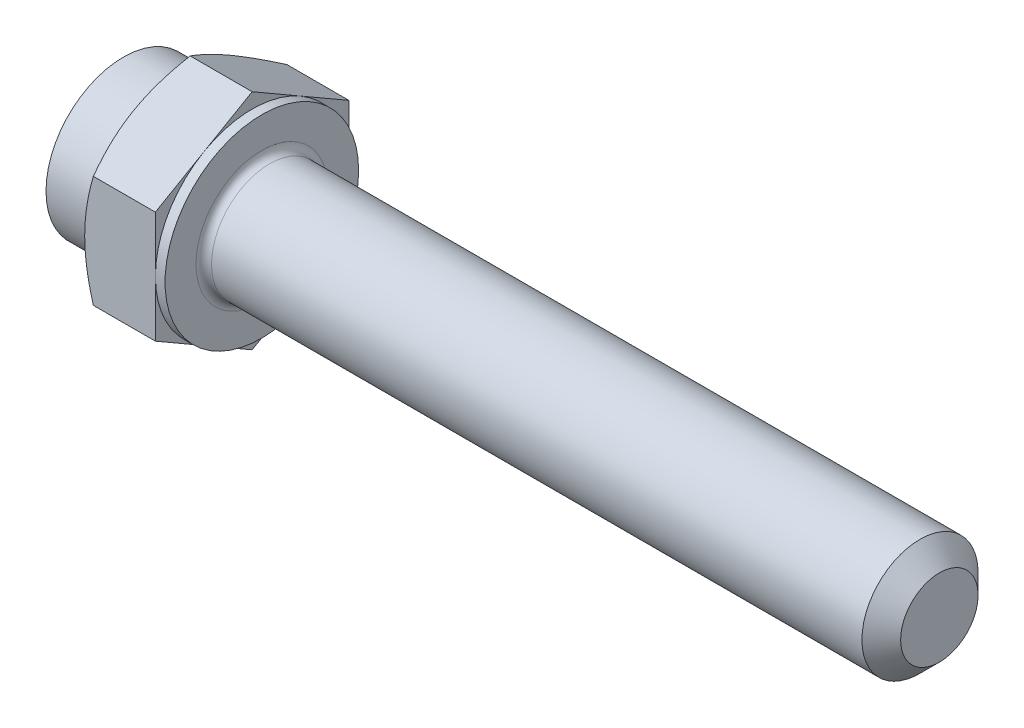
from build123d import *

# Parameters (mm, degrees)
EXTRUDE_371_DEPTH   = 4.15
SKETCH_4_W          = 0.5
SKETCH_4_H          = 10.773502692
CHAMFER_1937_SIZE   = 1
FILLET_1988_R       = 0.4
SKETCH_7_R          = 4
CUT_EXTRUDE_1_DEPTH = 3
SKETCH_8_R          = 4
EXTRUDE_1_DEPTH     = 6


with BuildPart() as part:
    # 草图1 → Extrude 371 (new body)
    with BuildSketch(Plane(origin=(0, 0, 0), x_dir=(0, 0, -1), z_dir=(1, 0, 0))):
        Polygon((5, 2.886751346), (5, -2.886751346), (0, -5.773502692), (-5, -2.886751346), (-5, 2.886751346), (0, 5.773502692), align=None)
    extrude(amount=EXTRUDE_371_DEPTH)

    # 草图2 → 凸台-旋转1 (revolve)
    with BuildSketch(Plane.XY, mode=Mode.PRIVATE) as revolve_1_sk:
        Polygon((0, 0), (39.15, 0), (39.15, 1.9175), (39.15, 3), (0, 3), align=None)
    revolve(revolve_1_sk.sketch.rotate(Axis((0, 0, 0), (1, 0, 0)), 90), axis=Axis((0, 0, 0), (1, 0, 0)))

    # 草图3 → 切除-旋转1 (revolve, cut)
    with BuildSketch(Plane.XY):
        Polygon((0, 5), (3.333333333, 10.773502692), (3.333333333, 15.773502692), (-10, 15.773502692), (-10, 5), align=None)
    revolve(axis=Axis((0, 0, 0), (1, 0, 0)), mode=Mode.SUBTRACT)

    # 草图5 → 切除-旋转2 (revolve, cut)
    with BuildSketch(Plane.XY):
        Polygon((4.15, 5), (0.816666667, 10.773502692), (0.816666667, 15.773502692), (10.816666667, 15.773502692), (10.816666667, 5), align=None)
    revolve(axis=Axis((0, 0, 0), (1, 0, 0)), mode=Mode.SUBTRACT)

    # 草图4 → 切除-旋转3 (revolve, cut)
    with BuildSketch(Plane.XY, mode=Mode.PRIVATE) as cut_revolve_3_sk:
        with Locations((3.9, 10.386751346)):
            Rectangle(SKETCH_4_W, SKETCH_4_H)
    revolve(cut_revolve_3_sk.sketch.rotate(Axis((0, 0, 0), (1, 0, 0)), 270), axis=Axis((0, 0, 0), (1, 0, 0)), mode=Mode.SUBTRACT)

    # Chamfer 1937
    chamfer_1937_edges = [part.edges().sort_by_distance(p)[0] for p in [
        (39.15, 0, -3),
    ]]
    chamfer(chamfer_1937_edges, length=CHAMFER_1937_SIZE)

    # Fillet 1988
    fillet_1988_edges = [part.edges().sort_by_distance(p)[0] for p in [
        (4.15, 0, -3),
    ]]
    fillet(fillet_1988_edges, radius=FILLET_1988_R)

    # 草图7 → 切除-拉伸1 (cut)
    with BuildSketch(Plane.ZY):
        Circle(SKETCH_7_R)
    extrude(amount=-CUT_EXTRUDE_1_DEPTH, mode=Mode.SUBTRACT)


with BuildPart() as body_2:
    # 草图8 → 凸台-拉伸1 (new body)
    with BuildSketch(Plane.ZY.offset(-3)):
        Circle(SKETCH_8_R)
    extrude(amount=EXTRUDE_1_DEPTH)


solid = Compound([part.part, body_2.part])
